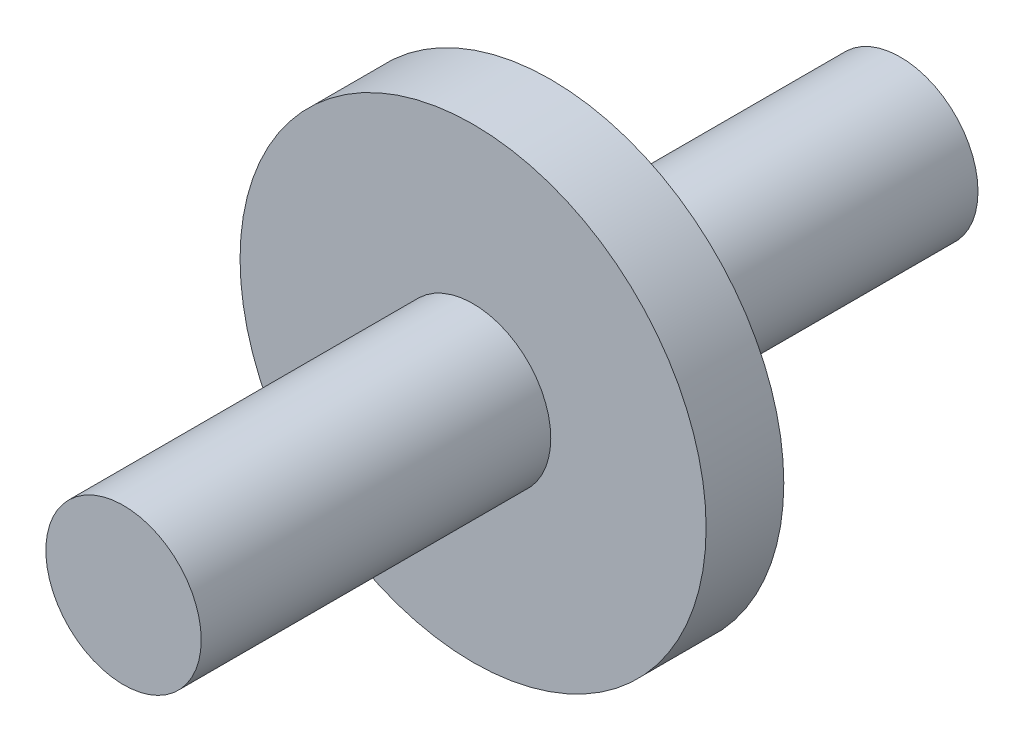
SolidWorks part; units mm, degrees
ref_plane "Front Plane" through (0, 0, 0) normal (0, 0, 1) x (1, 0, 0)
ref_plane "Top Plane" through (0, 0, 0) normal (0, 1, 0) x (1, 0, 0)
ref_plane "Right Plane" through (0, 0, 0) normal (1, 0, 0) x (0, 0, -1)
sketch "Sketch1" plane through (0, 0, 0) normal (0, 0, 1) x (1, 0, 0)
  circle A0 centre (0, 0) radius 40
  dimension "D1" = 80
extrude "Boss-Extrude1" add sketch "Sketch1" along normal mid plane 400
sketch "Sketch2" plane through (0, 0, 0) normal (0, 0, 1) x (1, 0, 0)
  circle A0 centre (0, 0) radius 120
  dimension "D1" = 240
extrude "Boss-Extrude2" add sketch "Sketch2" along normal mid plane 40
